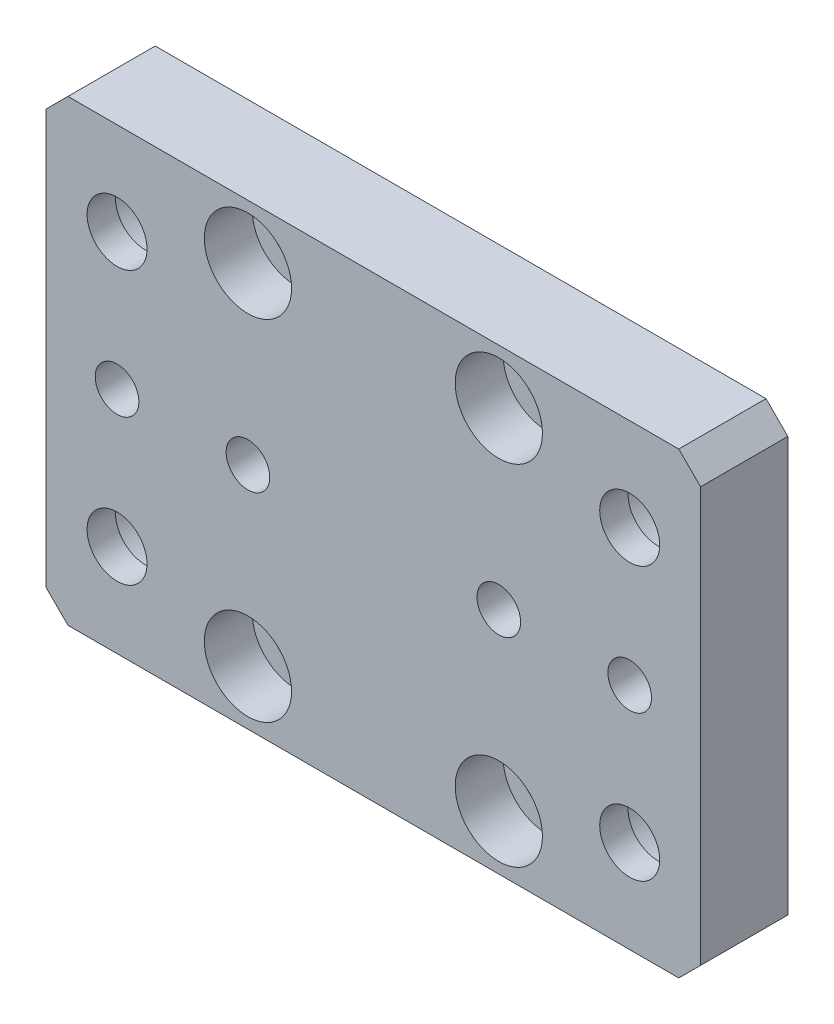
from build123d import *

# Parameters (mm, degrees)
SKETCH1_W                                           = 60
SKETCH1_H                                           = 42
BOSS_EXTRUDE1_DEPTH                                 = 8
CBORE_FOR_M4_HEX_SOCKET_HEAD_CAP_SCREW2_D           = 4.5
CBORE_FOR_M4_HEX_SOCKET_HEAD_CAP_SCREW2_CBORE_D     = 8
CBORE_FOR_M4_HEX_SOCKET_HEAD_CAP_SCREW2_CBORE_DEPTH = 4.4
SKETCH4_R                                           = 2
CUT_EXTRUDE1_DEPTH                                  = 74.674961826
CBORE_FOR_M5_HEX_SOCKET_HEAD_CAP_SCREW1_D           = 5.5
CBORE_FOR_M5_HEX_SOCKET_HEAD_CAP_SCREW1_CBORE_D     = 10
CBORE_FOR_M5_HEX_SOCKET_HEAD_CAP_SCREW1_CBORE_DEPTH = 5.4
SKETCH7_R                                           = 2
CUT_EXTRUDE2_DEPTH                                  = 74.674961826
CHAMFER1_SIZE                                       = 2


with BuildPart() as part:
    # Sketch1 → Boss-Extrude1 (new body)
    with BuildSketch(Plane.XY):
        with Locations((30, 21)):
            Rectangle(SKETCH1_W, SKETCH1_H)
    extrude(amount=BOSS_EXTRUDE1_DEPTH)

    # CBORE for M4 Hex Socket Head Cap Screw2 (through all)
    with Locations(Plane.XY.offset(8)):
        with Locations((41.5, 37), (18.5, 37), (18.5, 5), (41.5, 5)):
            CounterBoreHole(CBORE_FOR_M4_HEX_SOCKET_HEAD_CAP_SCREW2_D / 2, CBORE_FOR_M4_HEX_SOCKET_HEAD_CAP_SCREW2_CBORE_D / 2, CBORE_FOR_M4_HEX_SOCKET_HEAD_CAP_SCREW2_CBORE_DEPTH)

    # Sketch4 → Cut-Extrude1 (cut, through all)
    with BuildSketch(Plane.XY.offset(8)):
        with Locations((18.5, 21)):
            Circle(SKETCH4_R)
        with Locations((41.5, 21)):
            Circle(SKETCH4_R)
    extrude(amount=-CUT_EXTRUDE1_DEPTH, mode=Mode.SUBTRACT)

    # CBORE for M5 Hex Socket Head Cap Screw1 (through all)
    with Locations(Plane(origin=(0, 0, 0), x_dir=(1, 0, 0), z_dir=(0, 0, -1))):
        with Locations((53.5, -33.5), (6.5, -33.5), (6.5, -8.5), (53.5, -8.5)):
            CounterBoreHole(CBORE_FOR_M5_HEX_SOCKET_HEAD_CAP_SCREW1_D / 2, CBORE_FOR_M5_HEX_SOCKET_HEAD_CAP_SCREW1_CBORE_D / 2, CBORE_FOR_M5_HEX_SOCKET_HEAD_CAP_SCREW1_CBORE_DEPTH)

    # Sketch7 → Cut-Extrude2 (cut, through all)
    with BuildSketch(Plane.XY.offset(8)):
        with Locations((6.5, 21)):
            Circle(SKETCH7_R)
        with Locations(Location((53.5, 21, 0), (0, 0, 180))):
            Circle(SKETCH7_R)
    extrude(amount=-CUT_EXTRUDE2_DEPTH, mode=Mode.SUBTRACT)

    # Chamfer1
    chamfer1_edges = [part.edges().sort_by_distance(p)[0] for p in [
        (0, 42, 4),
        (60, 42, 4),
        (60, 0, 4),
        (0, 0, 4),
    ]]
    chamfer(chamfer1_edges, length=CHAMFER1_SIZE)


solid = part.part
